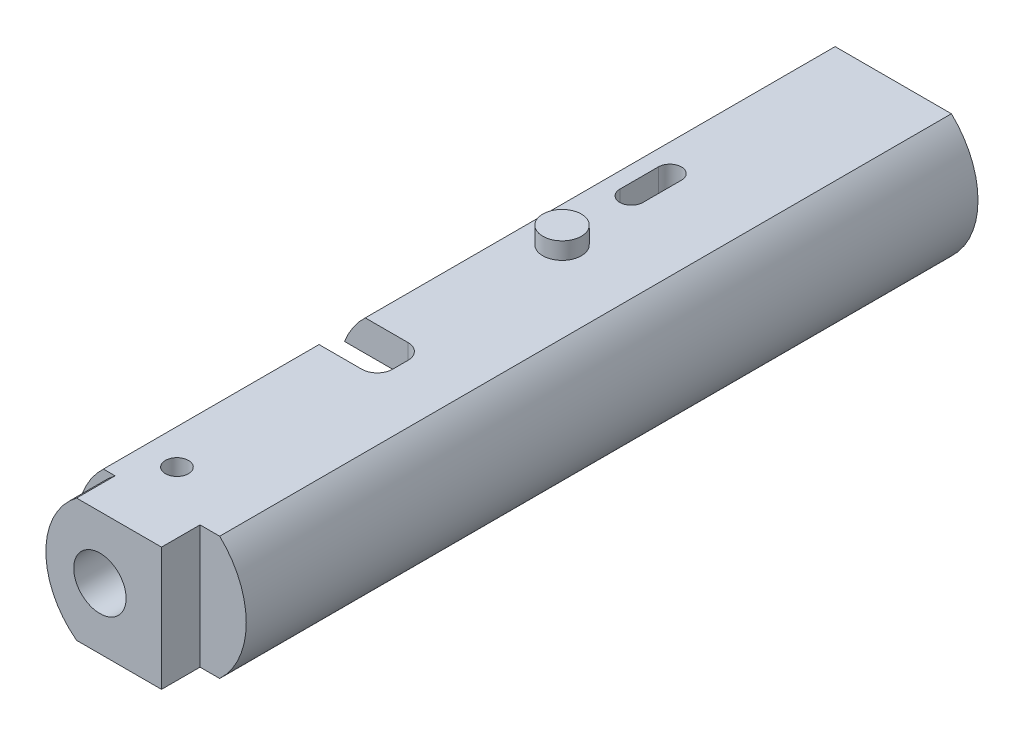
SolidWorks part; units mm, degrees
ref_plane "Front Plane" through (0, 0, 0) normal (0, 0, 1) x (1, 0, 0)
ref_plane "Top Plane" through (0, 0, 0) normal (0, 1, 0) x (1, 0, 0)
ref_plane "Right Plane" through (0, 0, 0) normal (1, 0, 0) x (0, 0, -1)
other "Configuration Table"
sketch "Sketch1" plane through (0, 0, 0) normal (0, 0, 1) x (1, 0, 0)
  circle A0 centre (0, 0) radius 11
  dimension "D1" = 22
extrude "Boss-Extrude1" add sketch "Sketch1" along normal blind 100
sketch "Sketch2" plane through (0, 0, 100) normal (0, 0, 1) x (1, 0, 0)
  line L0 (0, 0) -> (-11, 0) construction
  line L1 (-7.5498, 8) -> (7.5498, 8)
  line L2 (-7.5498, -8) -> (7.5498, -8)
  line L3 (-3, 0) -> (-3, 4.7088) construction
  circle A1 centre (0, 0) radius 11 construction
  arc A3 (7.5498, 8) -> (-7.5498, 8) centre (0, 0) ccw
  arc A4 (-7.5498, -8) -> (7.5498, -8) centre (0, 0) ccw
  dimension "D1" = 16
  dimension "D2" = 8
  dimension "D3" = 8
extrude "Cut-Extrude1" cut sketch "Sketch2" against normal through all
sketch "Sketch3" plane through (0, 0, 100) normal (0, 0, 1) x (1, 0, 0)
  circle A0 centre (-3, 0) radius 2
  arc A1 (-7.5498, 8) -> (-7.5498, -8) centre (0, 0) ccw construction
  dimension "D1" = 4
  dimension "D2" = 3
extrude "Cut-Extrude2" cut sketch "Sketch3" against normal blind 60
sketch "Sketch4" plane through (0, 0, 100) normal (0, 0, 1) x (1, 0, 0)
  line L0 (1, 4) -> (-12.898, 4)
  line L1 (-12.898, 4) -> (-12.898, -4)
  line L2 (-12.898, -4) -> (1, -4)
  line L3 (1, -4) -> (1, 4)
  circle A2 centre (-3, 0) radius 2 construction
  dimension "D1" = 1
  dimension "D2" = 8
  dimension "D3" = 4
extrude "Cut-Extrude3" cut sketch "Sketch4" against normal blind 65 from offset 15 offset against normal yes
sketch "Sketch5" plane through (0, -8, 0) normal (0, -1, 0) x (-1, 0, 0)
  line L7 (-5, -105) -> (-17, -105)
  line L8 (-5, -105) -> (-5, -95)
  line L9 (-5, -95) -> (-17, -95)
  line L10 (-17, -105) -> (-17, -95)
  line L11 (-5, -105) -> (-17, -95) construction
  line L12 (-5, -95) -> (-17, -105) construction
  point P6 (-11, -100)
  dimension "D2" = 10
extrude "Cut-Extrude4" cut sketch "Sketch5" against normal through all both and the other way through all
hole_wizard "M8 Tapped Hole1" positions "3DSketch1" profile "Sketch7" tap size "M8" standard "GB"
sketch3d "3DSketch1"
  line L0 (5, 8, 100) -> (5, -8, 100) construction
  point P0 (-3, -0.071, 100)
  dimension "D1" = 8
sketch "Sketch7" plane through (-3, -0.071, 100) normal (1, 0, 0) x (0, -1, 0)
  line L0 (0, 0) -> (0, 12.0429)
  line L1 (0, 12.0429) -> (3.4, 10)
  line L2 (3.4, 10) -> (3.4, 0)
  line L5 (3.4, 0) -> (0, 0)
  line L10 (0, 12.0429) -> (-3.4, 10) construction
  line L11 (0, -6.35) -> (0, 107.95) construction
  dimension "螺纹孔钻头直径" = 6.8
  dimension "螺纹孔钻头深度" = 10
  dimension "导头角度" = 118
cosmetic thread "Hole thread1" parameters "D1"=10, "D2"=8
sketch "Sketch8" plane through (0, -8, 0) normal (0, -1, 0) x (-1, 0, 0)
  line L2 (-5, -100) -> (7.5498, -100) construction
  line L3 (11, -100) -> (11, -85) construction
  circle A0 centre (3, -90) radius 1.5
  dimension "D1" = 3
  dimension "D2" = 8
  dimension "D3" = 10
extrude "Cut-Extrude5" cut sketch "Sketch8" against normal blind 3 and the other way through all
mirror "Mirror3" about plane through (0, 0, 0) normal (0, 1, 0) of "Cut-Extrude5"
sketch "Sketch9" plane through (0, -8, 0) normal (0, -1, 0) x (-1, 0, 0)
  line L0 (4, -30) -> (4, -25) construction
  line L1 (2.5, -30) -> (2.5, -25)
  line L2 (5.5, -30) -> (5.5, -25)
  line L4 (11, -20) -> (11, 0) construction
  line L5 (-7.5498, 0) -> (7.5498, 0) construction
  arc A0 (2.5, -30) -> (5.5, -30) centre (4, -30) ccw
  arc A1 (5.5, -25) -> (2.5, -25) centre (4, -25) ccw
  point P2 (4, -27.5)
  dimension "D3" = 25
  dimension "D1" = 5
  dimension "D2" = 3
  dimension "D4" = 7
extrude "Cut-Extrude6" cut sketch "Sketch9" against normal through all
sketch "Sketch10" plane through (0, 4, 0) normal (0, -1, 0) x (-1, 0, 0)
  line L0 (-7.5498, -95) -> (-5, -95) construction
  line L1 (2, -67) -> (19.8287, -67)
  line L2 (0, -65) -> (0, -63)
  line L3 (2, -61) -> (19.8287, -61)
  line L4 (19.8287, -67) -> (19.8287, -61)
  arc A0 (0, -63) -> (2, -61) centre (2, -63) cw
  arc A1 (2, -67) -> (0, -65) centre (2, -65) cw
  dimension "D3" = 2
  dimension "D1" = 28
  dimension "D2" = 34
extrude "Cut-Extrude7" cut sketch "Sketch10" against normal through all both and the other way through all
hole_wizard "M12x1.5 Tapped Hole1" positions "3DSketch2" profile "Sketch11" tap size "M12x1.5" standard "GB"
sketch3d "3DSketch2"
  line L0 (-7.5498, 8, 0) -> (7.5498, 8, 0) construction
  point P5 (0, 0, 0)
  dimension "D3" = 8
sketch "Sketch11" plane through (0, 0, 0) normal (1, 0, 0) x (0, 1, 0)
  line L0 (0, 0) -> (0, 22.6545)
  line L1 (0, 22.6545) -> (5.25, 19.5)
  line L2 (5.25, 19.5) -> (5.25, 0)
  line L5 (5.25, 0) -> (0, 0)
  line L10 (0, 22.6545) -> (-5.25, 19.5) construction
  line L11 (0, -6.35) -> (0, 107.95) construction
  dimension "螺纹孔钻头直径" = 10.5
  dimension "螺纹孔钻头深度" = 19.5
  dimension "导头角度" = 118
cosmetic thread "Hole thread5" parameters "D1"=15, "D2"=12
sketch "Sketch12" plane through (0, -8, 0) normal (0, -1, 0) x (1, 0, 0)
  line L1 (-3, 90) -> (-3, 40) construction
  circle A0 centre (-3, 40) radius 2.5
  circle A3 centre (-3, 90) radius 1.5 construction
  dimension "D1" = 5
  dimension "D2" = 50
extrude "Boss-Extrude2" add sketch "Sketch12" along normal blind 2.2
sketch "Sketch13" plane through (0, 8, 0) normal (0, 1, 0) x (1, 0, 0)
  circle A0 centre (-3, -40) radius 2.5
  circle A1 centre (-3, -90) radius 1.5 construction
  dimension "D1" = 50
  dimension "D2" = 5
extrude "Boss-Extrude3" add sketch "Sketch13" along normal blind 2.2
sketch "Sketch14" plane through (0, 0, 0) normal (0, 0, -1) x (-1, 0, 0)
  circle A0 centre (0, 0) radius 3.5
  dimension "D1" = 7
extrude "Cut-Extrude8" cut sketch "Sketch14" against normal blind 40
sketch "Sketch15" plane through (0, 0, 100) normal (0, 0, 1) x (1, 0, 0)
  circle A0 centre (0, 0) radius 10.0182
  circle A1 centre (0, 0) radius 14.7295
extrude "Cut-Extrude9" cut sketch "Sketch15" against normal blind 5
